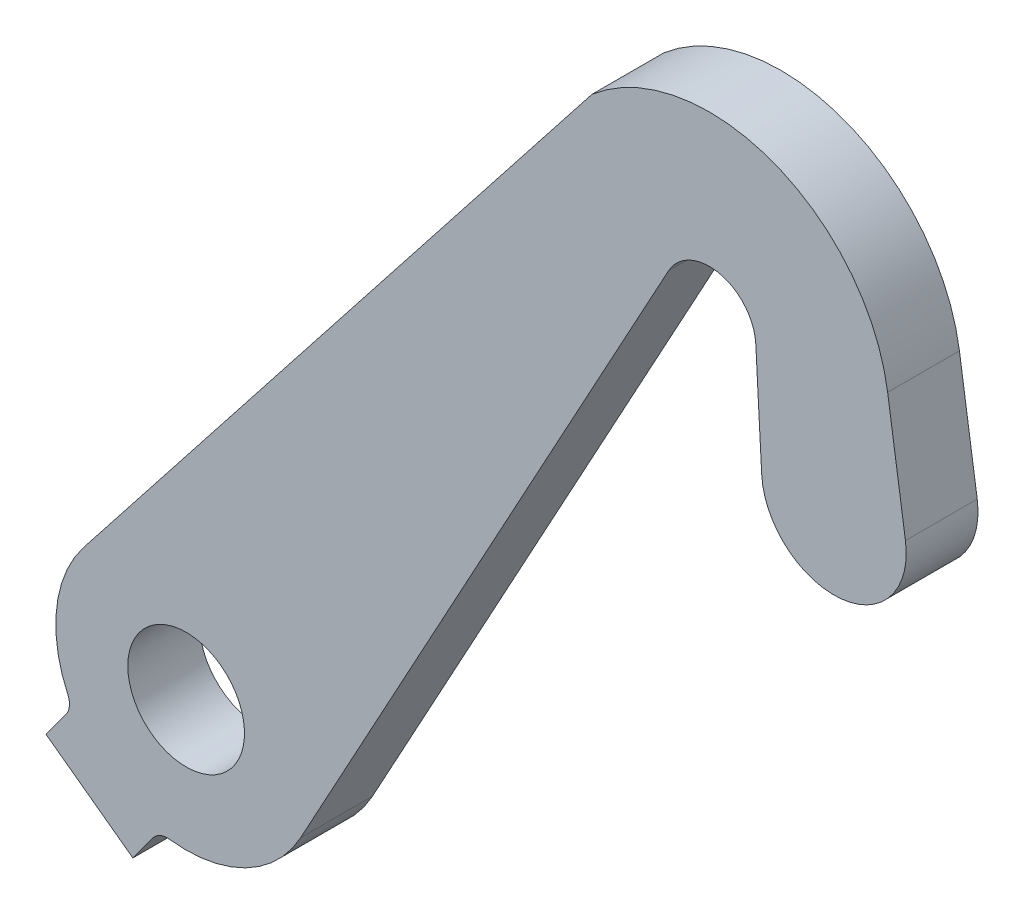
SolidWorks part; units mm, degrees
material "钢板5/Q235A "
ref_plane "Front Plane" through (0, 0, 0) normal (0, 0, 1) x (1, 0, 0)
ref_plane "Top Plane" through (0, 0, 0) normal (0, 1, 0) x (1, 0, 0)
ref_plane "Right Plane" through (0, 0, 0) normal (1, 0, 0) x (0, 0, -1)
sketch "Sketch1" plane through (0, 0, 0) normal (0, 0, 1) x (1, 0, 0)
  line L2 (47.6132, 66.5968) -> (6.6153, -8.6142)
  line L3 (57.9907, 52.1412) -> (57.3333, 64.3952)
  line L4 (-18.8001, -8.7844) -> (-21.756, -12.817)
  line L5 (-21.756, -12.817) -> (-12.0777, -19.9114)
  line L6 (-12.0777, -19.9114) -> (-9.1217, -15.8788)
  line L7 (-6.1395, -1.6615) -> (-12.9736, -10.9847) construction
  line L9 (58.8605, 88.3385) -> (-6.1395, -1.6615) construction
  line L10 (39.0763, 79.354) -> (-17.5594, 7.3168)
  line L11 (-6.1395, -1.6615) -> (58.8605, -1.6615) construction
  line L12 (58.8605, -1.6615) -> (58.8605, 88.3385) construction
  line L13 (74.008, 53.7594) -> (72.0258, 67.0748)
  arc A0 (-17.5594, 7.3168) -> (-18.8001, -8.7844) centre (-6.1395, -1.6615) ccw
  arc A1 (57.9907, 52.1412) -> (74.008, 53.7594) centre (66.0375, 52.5729) ccw
  arc A2 (57.3333, 64.3952) -> (47.6132, 66.5968) centre (52.161, 64.1177) ccw
  arc A4 (-9.1217, -15.8788) -> (6.6153, -8.6142) centre (-6.1395, -1.6615) ccw
  circle A5 centre (-6.1395, -1.6615) radius 6.5
  arc A11 (72.0258, 67.0748) -> (39.0763, 79.354) centre (52.161, 64.1177) ccw
  dimension "D3" = 13
  dimension "D5" = 65
  dimension "D1" = 12
  dimension "D2" = 5
  dimension "D6" = 90
extrude "Boss-Extrude1" add sketch "Sketch1" along normal mid plane 8
fillet "Fillet1" radius 2 2 edges at (-9.1217, -15.8788, 0) (-18.8001, -8.7844, 0)
